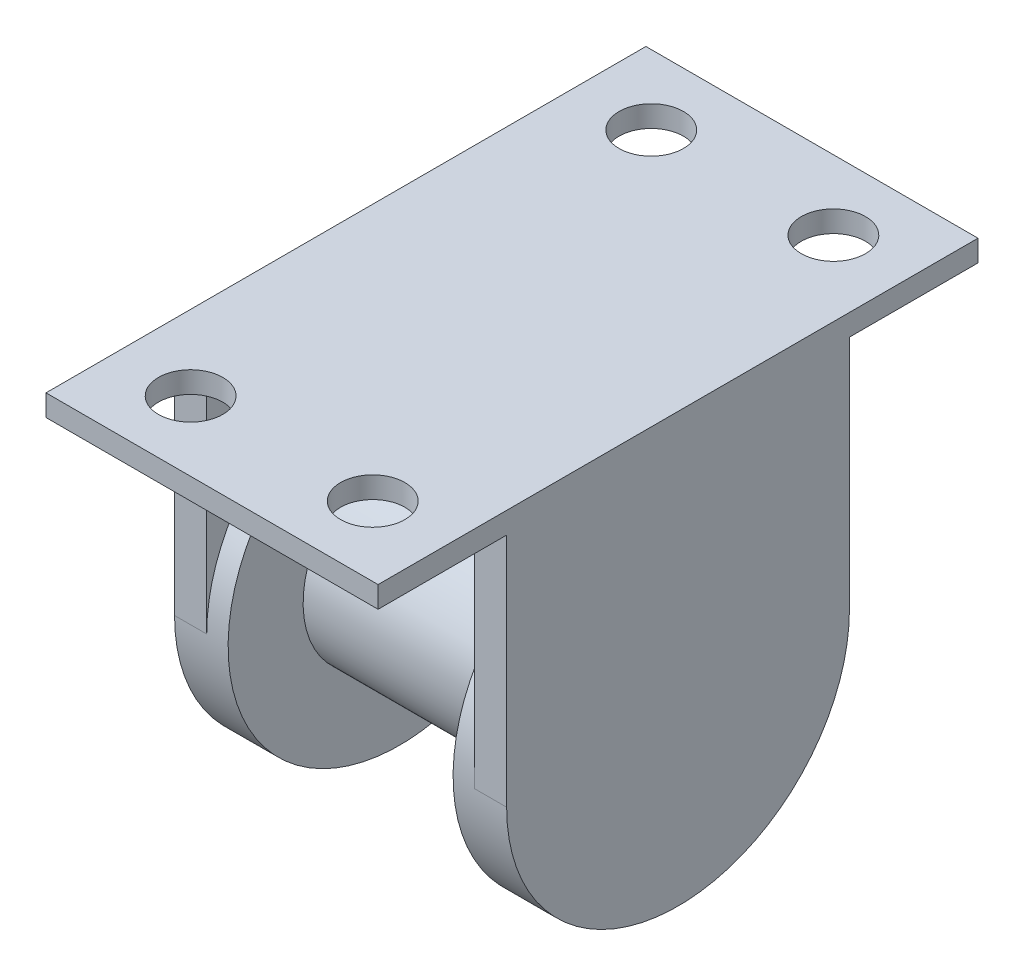
from build123d import *

# Parameters (mm, degrees)
EXTRUDE_START       = 3
EXTRUDE_1_DEPTH     = 3
SKETCH_4_W          = 31
SKETCH_4_H          = 2
EXTRUDE_2_DEPTH     = 28
CUT_EXTRUDE_1_REACH = 58.285
SKETCH_5_R          = 3


with BuildPart() as part:
    # 草图1 → 旋转1 (revolve)
    with BuildSketch(Plane.XY):
        Polygon((2, 16), (0, 16), (0, 0), (25, 0), (25, 16), (23, 16), (23, 9), (2, 9), align=None)
    revolve(axis=Axis((25, 0, 0), (-1, 0, 0)))

    # 草图2 → 凸台-拉伸1 (add)
    with BuildSketch(Plane.ZY.offset(EXTRUDE_START)):
        with BuildLine():
            Line((-16, 0), (-16, 24))
            Line((-16, 24), (16, 24))
            Line((16, 24), (16, 0))
            ThreePointArc((16, 0), (0, -16), (-16, 0))
        make_face()
    extrude_1 = extrude(amount=-EXTRUDE_1_DEPTH)

    # 镜向1: 凸台-拉伸1 across plane
    add(extrude_1.mirror(Plane(origin=(12.5, 0, 0), x_dir=(0, 0, 1), z_dir=(1, 0, 0))))

    # 草图4 → 凸台-拉伸2 (add, symmetric)
    with BuildSketch(Plane.XY):
        with Locations((12.5, 23)):
            Rectangle(SKETCH_4_W, SKETCH_4_H)
    extrude(amount=EXTRUDE_2_DEPTH, both=True)

    # 草图5 → 切除-拉伸1 (cut, up to next)
    with BuildSketch(Plane(origin=(0, 24, 0), x_dir=(1, 0, 0), z_dir=(0, 1, 0)), mode=Mode.PRIVATE) as cut_extrude_1_sk1:
        with Locations(Location((4, 21.5, 0), (0, 0, 180))):
            Circle(SKETCH_5_R)
    cut_extrude_1_tool1 = extrude(cut_extrude_1_sk1.sketch, amount=-CUT_EXTRUDE_1_REACH, mode=Mode.PRIVATE) & part.part
    # 草图5 → 切除-拉伸1 (cut, up to next)
    with BuildSketch(Plane(origin=(0, 24, 0), x_dir=(1, 0, 0), z_dir=(0, 1, 0)), mode=Mode.PRIVATE) as cut_extrude_1_sk2:
        with Locations(Location((4, -21.5, 0), (0, 0, 270))):
            Circle(SKETCH_5_R)
    cut_extrude_1_tool2 = extrude(cut_extrude_1_sk2.sketch, amount=-CUT_EXTRUDE_1_REACH, mode=Mode.PRIVATE) & part.part
    # 草图5 → 切除-拉伸1 (cut, up to next)
    with BuildSketch(Plane(origin=(0, 24, 0), x_dir=(1, 0, 0), z_dir=(0, 1, 0)), mode=Mode.PRIVATE) as cut_extrude_1_sk3:
        with Locations(Location((21, -21.5, 0), (0, 0, 180))):
            Circle(SKETCH_5_R)
    cut_extrude_1_tool3 = extrude(cut_extrude_1_sk3.sketch, amount=-CUT_EXTRUDE_1_REACH, mode=Mode.PRIVATE) & part.part
    # 草图5 → 切除-拉伸1 (cut, up to next)
    with BuildSketch(Plane(origin=(0, 24, 0), x_dir=(1, 0, 0), z_dir=(0, 1, 0)), mode=Mode.PRIVATE) as cut_extrude_1_sk4:
        with Locations(Location((21, 21.5, 0), (0, 0, 270))):
            Circle(SKETCH_5_R)
    cut_extrude_1_tool4 = extrude(cut_extrude_1_sk4.sketch, amount=-CUT_EXTRUDE_1_REACH, mode=Mode.PRIVATE) & part.part
    add(cut_extrude_1_tool1.solids().sort_by_distance((4, 24, -21.5))[0], mode=Mode.SUBTRACT)
    add(cut_extrude_1_tool2.solids().sort_by_distance((4, 24, 21.5))[0], mode=Mode.SUBTRACT)
    add(cut_extrude_1_tool3.solids().sort_by_distance((21, 24, 21.5))[0], mode=Mode.SUBTRACT)
    add(cut_extrude_1_tool4.solids().sort_by_distance((21, 24, -21.5))[0], mode=Mode.SUBTRACT)


solid = part.part
